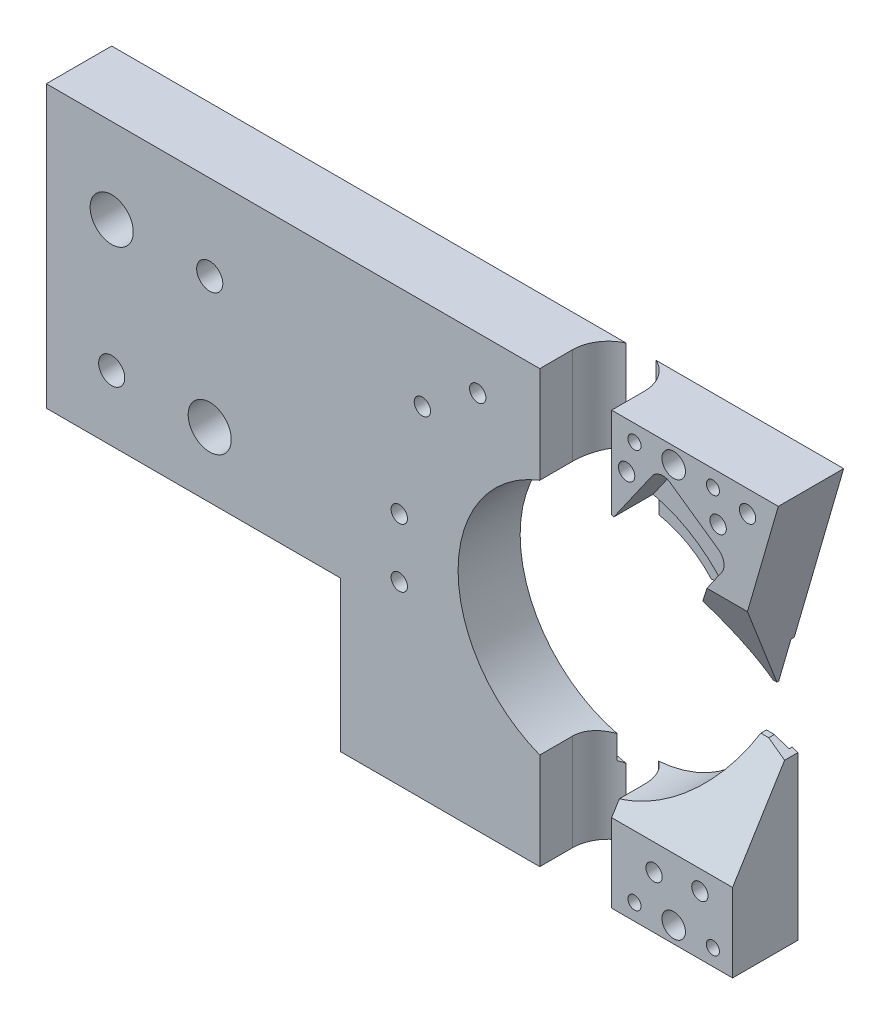
from build123d import *

# Parameters (mm, degrees)
EXTRUDE_1_DEPTH     = 10
CUT_EXTRUDE_2_DEPTH = 89.50641067
CUT_EXTRUDE_3_DEPTH = 73.982084992
CUT_EXTRUDE_4_DEPTH = 56
SKETCH_7_R          = 23
CUT_EXTRUDE_5_DEPTH = 0.5
SKETCH_8_R          = 19.5
CUT_EXTRUDE_6_DEPTH = 8.5
CUT_EXTRUDE_7_DEPTH = 8
SKETCH_10_R         = 2
SKETCH_10_R_2       = 3.3
SKETCH_10_R_3       = 1.25
SKETCH_10_R_4       = 1
SKETCH_10_R_5       = 1.8
SKETCH_10_R_6       = 0.8
CUT_EXTRUDE_8_DEPTH = 73.982085064
CUT_EXTRUDE_9_DEPTH = 6


with BuildPart() as part:
    # 草图1 → 凸台-拉伸1 (new body)
    with BuildSketch(Plane.XY):
        Polygon((-53.884728945, 0), (-8.884728945, 0), (-8.884728945, -23), (58.115271055, -23), (58.115271055, 43), (-53.884728945, 43), align=None)
    extrude(amount=EXTRUDE_1_DEPTH)

    # 草图3 → 切除-拉伸2 (cut, through all)
    with BuildSketch(Plane.XZ.offset(23)):
        with BuildLine():
            Line((32.615271055, 5), (32.615271055, 10))
            Line((32.615271055, 10), (21.615271055, 10))
            Line((21.615271055, 10), (21.615271055, 5))
            ThreePointArc((21.615271055, 5), (27.115271055, -0.5), (32.615271055, 5))
        make_face()
    extrude(amount=-CUT_EXTRUDE_2_DEPTH, mode=Mode.SUBTRACT)


with BuildPart() as cut_extrude_2_piece_1:
    # of the separate pieces the step leaves, piece 1, a body of its own (cut_extrude_2_pieces)
    add(part.part.solids().sort_by_distance((-53.884728945, 0, 0))[0])


with BuildPart() as cut_extrude_2_piece_2:
    # of the separate pieces the step leaves, piece 2, a body of its own (cut_extrude_2_pieces)
    add(part.part.solids().sort_by_distance((58.115271055, 43, 0))[0])

    # 草图4 → 切除-拉伸3 (cut, through all)
    with BuildSketch(Plane(origin=(0, 0, 0), x_dir=(-1, 0, 0), z_dir=(0, 0, -1))):
        Polygon((-58.115271055, -23), (-58.115271055, 43), (-48.419070628, 9.488742909), (-45.499700026, 10), (-44.487463913, 4.219948433), (-51.115271055, 1.87), (-51.115271055, -23), align=None)
    extrude(amount=-CUT_EXTRUDE_3_DEPTH, mode=Mode.SUBTRACT)

    # 草图6 → 切除-拉伸4 (cut)
    with BuildSketch(Plane(origin=(80, 0, 0), x_dir=(0, 0, -1), z_dir=(1, 0, 0))):
        Polygon((-10, 26.69), (-0.78, 10.37), (0, 10.37), (0, 2.97), (-1.36, 2.97), (-10, -11), align=None)
    extrude(amount=-CUT_EXTRUDE_4_DEPTH, mode=Mode.SUBTRACT)


with BuildPart() as cut_extrude_4_piece_1:
    # of the separate pieces the step leaves, piece 1, a body of its own (cut_extrude_4_pieces)
    add(cut_extrude_2_piece_2.part.solids().sort_by_distance((58.115271055, 43, 0))[0])


with BuildPart() as cut_extrude_4_piece_2:
    # of the separate pieces the step leaves, piece 2, a body of its own (cut_extrude_4_pieces)
    add(cut_extrude_2_piece_2.part.solids().sort_by_distance((48.012825165, 2.97, 0))[0])


with BuildPart() as cut_extrude_5_tool:
    # 草图7 → 切除-拉伸5 (new body)
    with BuildSketch(Plane(origin=(0, 0, 0), x_dir=(-1, 0, 0), z_dir=(0, 0, -1))):
        with Locations((-28.615271055, 10)):
            Circle(SKETCH_7_R)
    extrude(amount=-CUT_EXTRUDE_5_DEPTH)


with BuildPart() as cut_extrude_2_piece_1_1:
    add(cut_extrude_2_piece_1.part)

    # 切除-拉伸5: cut by cut_extrude_5_tool
    add(cut_extrude_5_tool.part, mode=Mode.SUBTRACT)


with BuildPart() as cut_extrude_4_piece_1_1:
    add(cut_extrude_4_piece_1.part)

    # 切除-拉伸5: cut by cut_extrude_5_tool
    add(cut_extrude_5_tool.part, mode=Mode.SUBTRACT)


with BuildPart() as cut_extrude_4_piece_2_1:
    add(cut_extrude_4_piece_2.part)

    # 切除-拉伸5: cut by cut_extrude_5_tool
    add(cut_extrude_5_tool.part, mode=Mode.SUBTRACT)


with BuildPart() as cut_extrude_6_tool:
    # 草图8 → 切除-拉伸6 (new body)
    with BuildSketch(Plane.XY.offset(10)):
        with Locations((28.615271055, 10)):
            Circle(SKETCH_8_R)
    extrude(amount=-CUT_EXTRUDE_6_DEPTH)


with BuildPart() as cut_extrude_2_piece_1_2:
    add(cut_extrude_2_piece_1_1.part)

    # 切除-拉伸6: cut by cut_extrude_6_tool
    add(cut_extrude_6_tool.part, mode=Mode.SUBTRACT)


with BuildPart() as cut_extrude_4_piece_1_2:
    add(cut_extrude_4_piece_1_1.part)

    # 切除-拉伸6: cut by cut_extrude_6_tool
    add(cut_extrude_6_tool.part, mode=Mode.SUBTRACT)


with BuildPart() as cut_extrude_4_piece_2_2:
    add(cut_extrude_4_piece_2_1.part)

    # 切除-拉伸6: cut by cut_extrude_6_tool
    add(cut_extrude_6_tool.part, mode=Mode.SUBTRACT)


with BuildPart() as cut_extrude_7_tool:
    # 草图9 → 切除-拉伸7 (new body)
    with BuildSketch(Plane(origin=(0, 0, 0), x_dir=(-1, 0, 0), z_dir=(0, 0, -1))):
        with BuildLine():
            Line((-39.359635932, 19.736971983), (-45.069748889, 20.464232375))
            ThreePointArc((-45.069748889, 20.464232375), (-18.354208401, -6.58193575), (-30.637865502, 29.394821775))
            Line((-30.637865502, 29.394821775), (-30.637865502, 24.358241943))
            ThreePointArc((-30.637865502, 24.358241943), (-35.404074087, 22.812577937), (-39.359635932, 19.736971983))
        make_face()
    extrude(amount=-CUT_EXTRUDE_7_DEPTH)


with BuildPart() as cut_extrude_2_piece_1_3:
    add(cut_extrude_2_piece_1_2.part)

    # 切除-拉伸7: cut by cut_extrude_7_tool
    add(cut_extrude_7_tool.part, mode=Mode.SUBTRACT)


with BuildPart() as cut_extrude_4_piece_1_3:
    add(cut_extrude_4_piece_1_2.part)

    # 切除-拉伸7: cut by cut_extrude_7_tool
    add(cut_extrude_7_tool.part, mode=Mode.SUBTRACT)


with BuildPart() as cut_extrude_4_piece_2_3:
    add(cut_extrude_4_piece_2_2.part)

    # 切除-拉伸7: cut by cut_extrude_7_tool
    add(cut_extrude_7_tool.part, mode=Mode.SUBTRACT)


with BuildPart() as cut_extrude_8_tool:
    # 草图10 → 切除-拉伸8 (new, through all)
    with BuildSketch(Plane(origin=(0, 0, 0), x_dir=(-1, 0, 0), z_dir=(0, 0, -1))):
        with Locations((43.884728945, 10)):
            Circle(SKETCH_10_R)
        with Locations((28.884728945, 10)):
            Circle(SKETCH_10_R_2)
        with Locations((28.884728945, 30)):
            Circle(SKETCH_10_R)
        with Locations((43.884728945, 30)):
            Circle(SKETCH_10_R_2)
        with Locations((-0.115271055, 4)):
            Circle(SKETCH_10_R_3)
        with Locations((-0.115271055, 13)):
            Circle(SKETCH_10_R_3)
        with Locations((-3.652993394, 29)):
            Circle(SKETCH_10_R_3)
        with Locations((-12.123983207, 35)):
            Circle(SKETCH_10_R_3)
        with Locations((-48.106558902, -20.5)):
            Circle(SKETCH_10_R_4)
        with Locations((-42.106558902, -20.5)):
            Circle(SKETCH_10_R_5)
        with Locations((-36.106558902, -20.5)):
            Circle(SKETCH_10_R_4)
        with Locations((-46.115271055, -14)):
            Circle(SKETCH_10_R_3)
        with Locations((-39.106558902, -14.996384308)):
            Circle(SKETCH_10_R_3)
        with Locations((-34.906558902, 36)):
            Circle(SKETCH_10_R_3)
        with Locations((-36.106558902, 40.5)):
            Circle(SKETCH_10_R_4)
        with Locations((-41.406558902, 34.99113626)):
            Circle(SKETCH_10_R_6)
        with Locations((-42.106558902, 40.5)):
            Circle(SKETCH_10_R_5)
        with Locations((-48.906558902, 36)):
            Circle(SKETCH_10_R_3)
        with Locations((-46.477548715, 31.5)):
            Circle(SKETCH_10_R_6)
        with Locations((-48.106558902, 40.5)):
            Circle(SKETCH_10_R_4)
        with Locations((-53.406558902, 39.65)):
            Circle(SKETCH_10_R_3)
    extrude(amount=-CUT_EXTRUDE_8_DEPTH)


with BuildPart() as cut_extrude_2_piece_1_4:
    add(cut_extrude_2_piece_1_3.part)

    # 切除-拉伸8: cut by cut_extrude_8_tool
    add(cut_extrude_8_tool.part, mode=Mode.SUBTRACT)


with BuildPart() as cut_extrude_4_piece_1_4:
    add(cut_extrude_4_piece_1_3.part)

    # 切除-拉伸8: cut by cut_extrude_8_tool
    add(cut_extrude_8_tool.part, mode=Mode.SUBTRACT)

    # 草图11 → 切除-拉伸9 (cut)
    with BuildSketch(Plane.XY.offset(10)):
        with BuildLine():
            Line((32.948740967, 29.01239171), (38.799220617, 37.367742561))
            ThreePointArc((38.799220617, 37.367742561), (40.090228351, 38.190205195), (41.584677579, 37.858893777))
            Line((41.584677579, 37.858893777), (48.957045977, 32.69670585))
            ThreePointArc((48.957045977, 32.69670585), (49.77950861, 31.405698117), (49.448197193, 29.911248889))
            Line((49.448197193, 29.911248889), (43.94502872, 22.051909804))
            ThreePointArc((43.94502872, 22.051909804), (39.044686512, 26.476568005), (32.948740967, 29.01239171))
        make_face()
    extrude(amount=-CUT_EXTRUDE_9_DEPTH, mode=Mode.SUBTRACT)


with BuildPart() as cut_extrude_4_piece_2_4:
    add(cut_extrude_4_piece_2_3.part)

    # 切除-拉伸8: cut by cut_extrude_8_tool
    add(cut_extrude_8_tool.part, mode=Mode.SUBTRACT)


solid = Compound([cut_extrude_2_piece_1_4.part, cut_extrude_4_piece_1_4.part, cut_extrude_4_piece_2_4.part])
